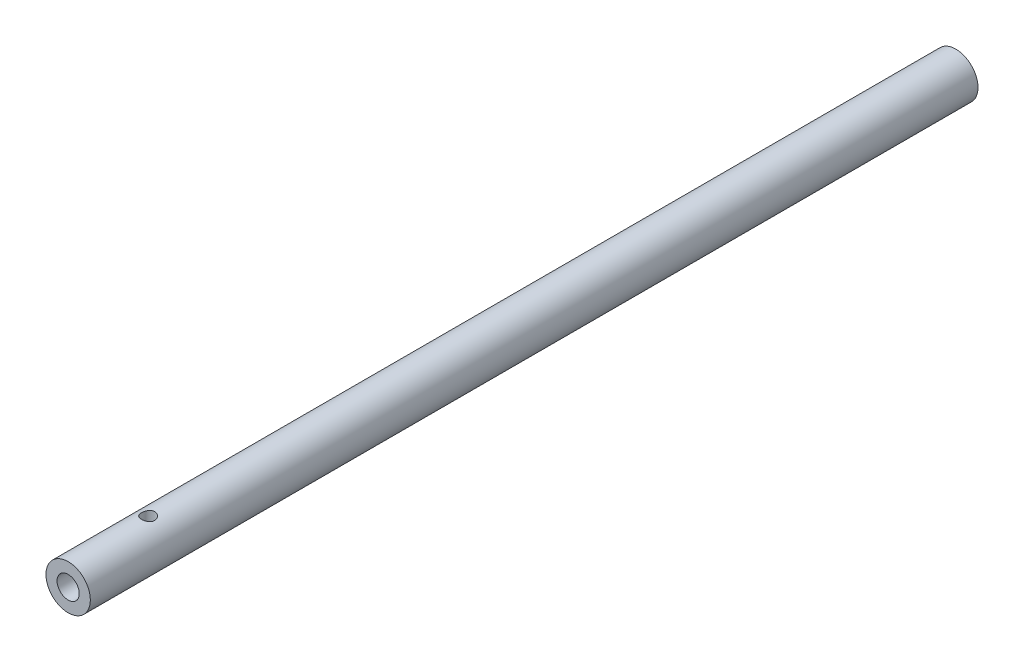
SolidWorks part; units mm, degrees
ref_plane "Front Plane" through (0, 0, 0) normal (0, 0, 1) x (1, 0, 0)
ref_plane "Top Plane" through (0, 0, 0) normal (0, 1, 0) x (1, 0, 0)
ref_plane "Right Plane" through (0, 0, 0) normal (1, 0, 0) x (0, 0, -1)
other "Configuration Table"
sketch "Sketch2" plane through (0, 0, 0) normal (0, 0, 1) x (1, 0, 0)
  circle A0 centre (0, 0) radius 2.5
  circle A1 centre (0, 0) radius 1.25
  dimension "D1" = 5
  dimension "D2" = 2.5
extrude "Boss-Extrude1" add sketch "Sketch2" along normal blind 100
ref_plane "Plane1" through (0, 2.5, 0) normal (0, 1, 0) x (1, 0, 0)
sketch "Sketch3" plane through (0, 2.5, 0) normal (0, 1, 0) x (1, 0, 0)
  line L0 (2.5, 0) -> (-2.5, 0) construction
  line L1 (-2.5, 0) -> (-2.5, -100) construction
  circle A0 centre (0, -91) radius 0.75
  dimension "D1" = 1.5
  dimension "D2" = 91
  dimension "D3" = 2.5
extrude "Cut-Extrude1" cut sketch "Sketch3" against normal up to surface (1.25 mm away)
